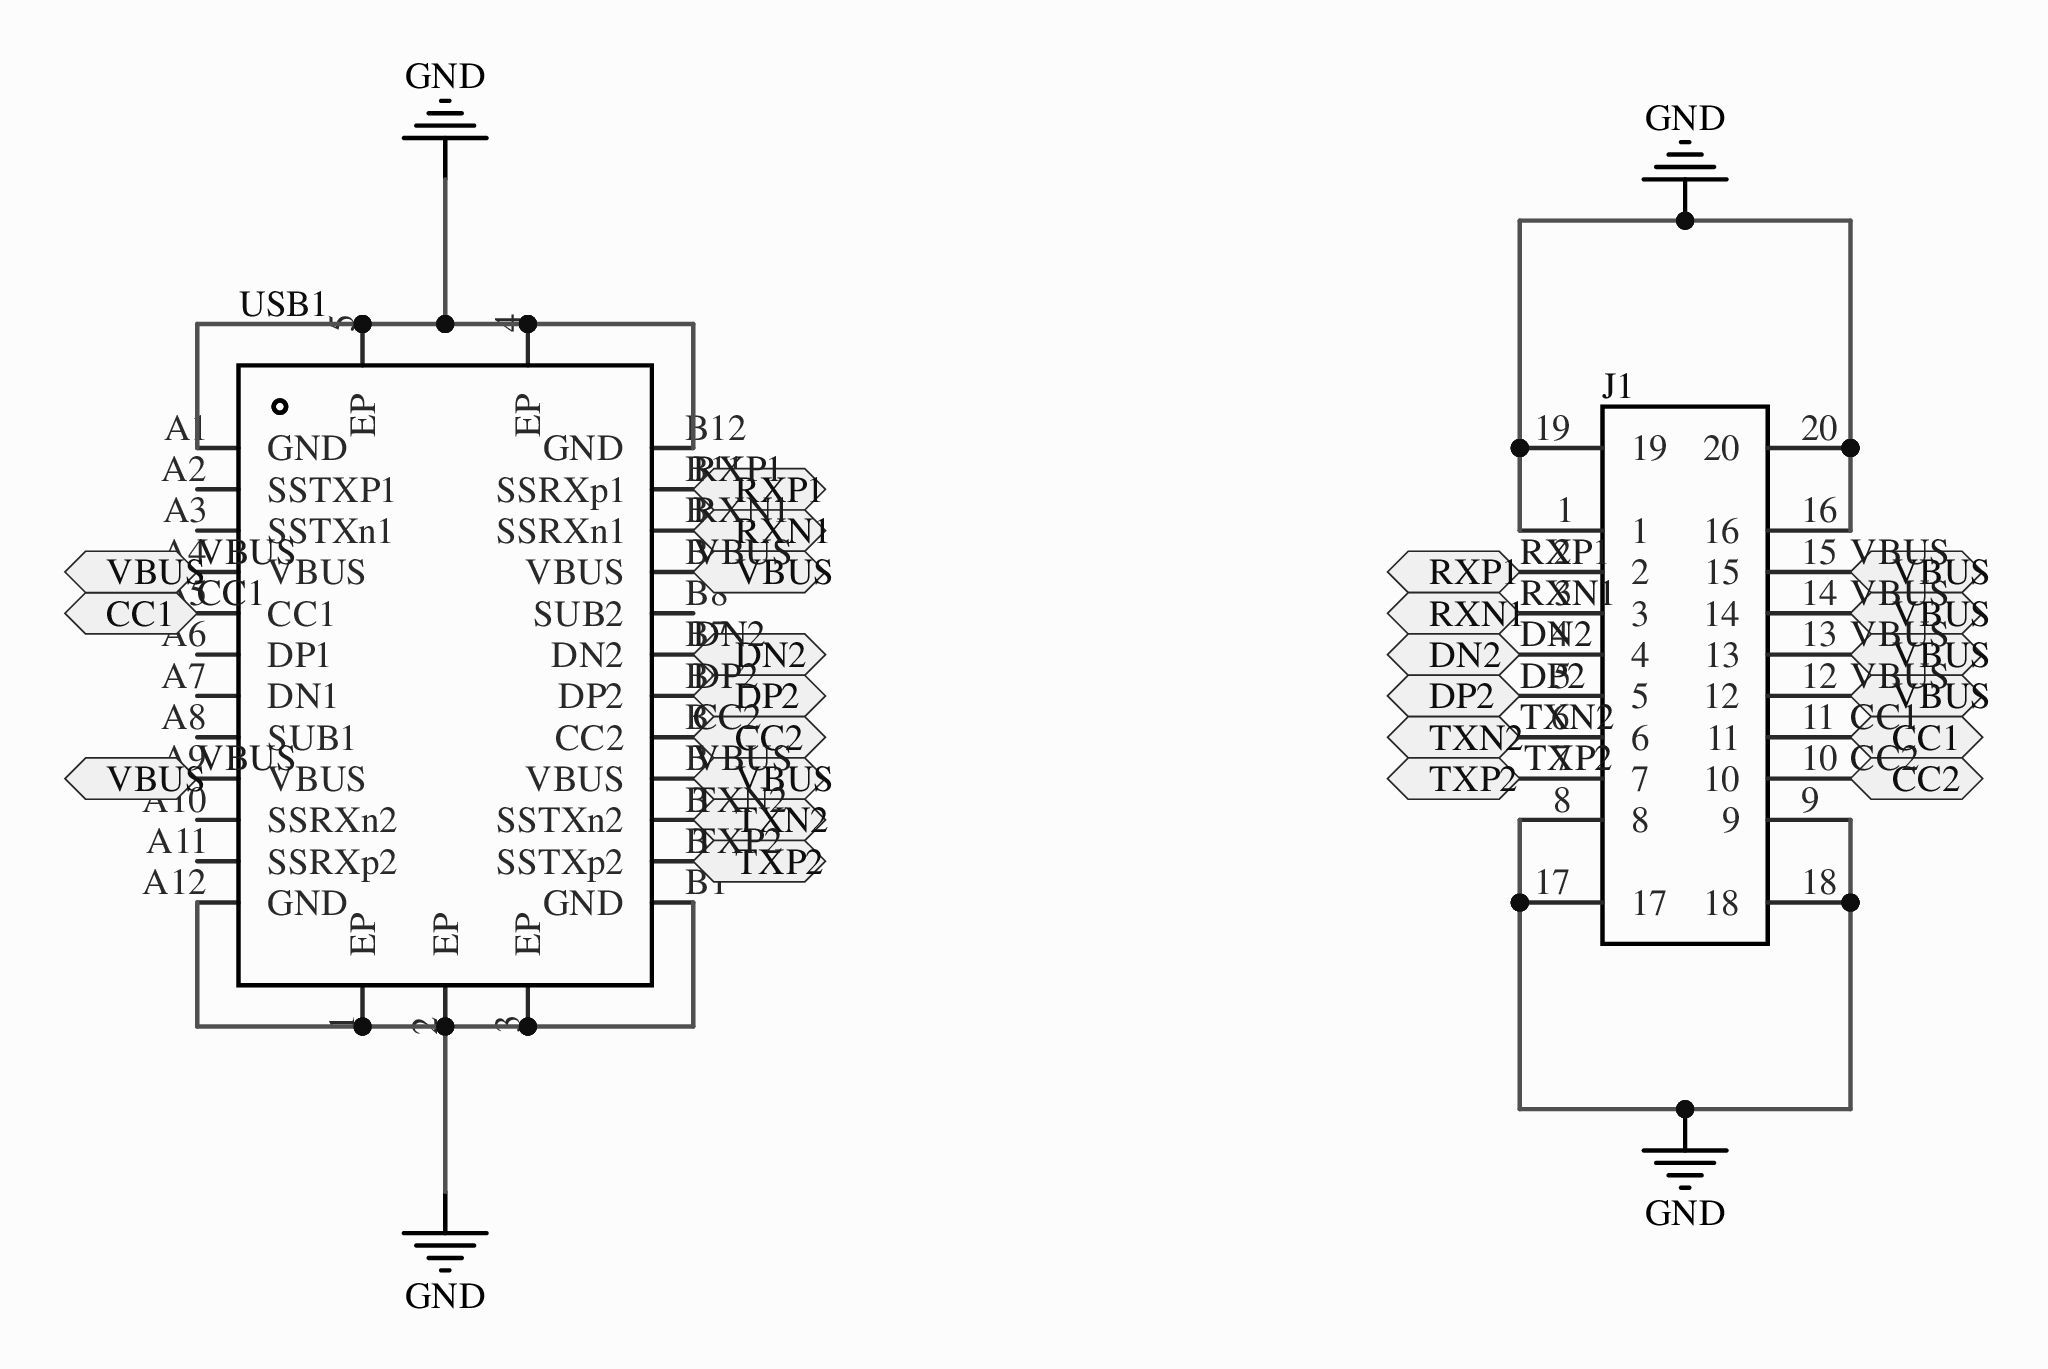
[diagram p0: MISC89352-2.schdoc]
# Altium project MISC89352-12.PrjPCB
1 sheet, 2 parts. Net scope: flat (ports and power ports of the same name join across sheets).
Board file: MISC89352.pcbdoc

## Sheet MISC89352-2.schdoc
size 320 x 236 mm; Version: V1.0; @Project Name: MISC89352; @Page Count: 1; @Update Date: 2024-04-23; @Create Date: 2024-04-23; @Schematic Name: MISC89352; @Page No: 1

### Parts
J1  BK13C06-16DS  [BK13C06-16DS_AA]  (value not drawn)
USB1  TYPEC-952-ACP24  [USB-C-SMD_TYPEC-952-ACP24]  (value not drawn)

### Ports
CC1 (bidir), CC2 (bidir), DN2 (bidir), DP2 (bidir), RXN1 (bidir), RXP1 (bidir), TXN2 (bidir), TXP2 (bidir), VBUS (bidir)

### Nets
GND: J1.1 J1.8 J1.9 J1.16 J1.17 J1.18 J1.19 J1.20 USB1.1(EP) USB1.2(EP) USB1.3(EP) USB1.4(EP) USB1.5(EP) USB1.A1(GND) USB1.A12(GND) USB1.B1(GND) USB1.B12(GND)
CC1: J1.11 USB1.A5(CC1) ; port CC1
CC2: J1.10 USB1.B5(CC2) ; port CC2
DN2: J1.4 USB1.B7(DN2) ; port DN2
DP2: J1.5 USB1.B6(DP2) ; port DP2
RXN1: J1.3 USB1.B10(SSRXn1) ; port RXN1
RXP1: J1.2 USB1.B11(SSRXp1) ; port RXP1
TXN2: J1.6 USB1.B3(SSTXn2) ; port TXN2
TXP2: J1.7 USB1.B2(SSTXp2) ; port TXP2
VBUS: J1.12 J1.13 J1.14 J1.15 USB1.A4(VBUS) USB1.A9(VBUS) USB1.B4(VBUS) USB1.B9(VBUS) ; port VBUS

Not connected (* = marked no-connect by the designer): USB1 A2(SSTXP1)* A3(SSTXn1) A6(DP1)* A7(DN1)* A8(SUB1)* A10(SSRXn2)* A11(SSRXp2)* B8(SUB2)*

### Notes on the sheet
- Labels drawn without touching a wire or pin: TXP2
- 1
- A

### Library data of the parts
J1 = BK13C06-16DS: 2-0.35V(800); Add into BOM: yes; Name: BK13C06-16DS; Symbol: BK13C06-16DS; Device: BK13C06-16DS; Convert to PCB: yes; Origin Footprint 2: BK13C06-16DS_AA; Origin Footprint 1: BK13C06-16DS
USB1 = TYPEC-952-ACP24: Add into BOM: yes; Connector Type: Type-C; Number of Ports: 1; Number of Contacts: 24P; Current Rating - Power (Max): 5A; Name: TYPEC-952-ACP24; Symbol: TYPEC-952-ACP24; Device: TYPEC-952-ACP24; Supplier: LCSC; Supplier Part: C2840398; Manufacturer Part: TYPEC-952-ACP24; Supplier Footprint: SMD; Datasheet: https://atta.szlcsc.com/upload/public/pdf/source/20210621/C2840398_046BEFA6439807122D1E5D18F63836BA.pdf; Convert to PCB: yes; Standard: USB 3.1; Origin Footprint 2: USB-C-SMD_TYPEC-952-ACP24; Origin Footprint 1: TYPEC-952-ACP24